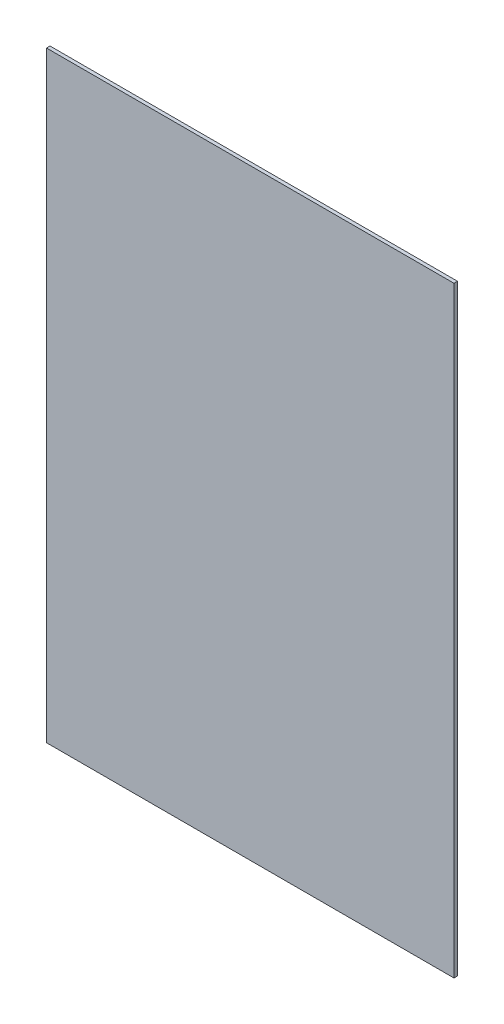
from build123d import *

# Parameters (mm, degrees)
SKETCH_1_W      = 581
SKETCH_1_H      = 858
EXTRUDE_1_DEPTH = 5


with BuildPart() as part:
    # 草图1 → 凸台-拉伸1 (new body)
    with BuildSketch(Plane.XY):
        Rectangle(SKETCH_1_W, SKETCH_1_H)
    extrude(amount=EXTRUDE_1_DEPTH)


solid = part.part
